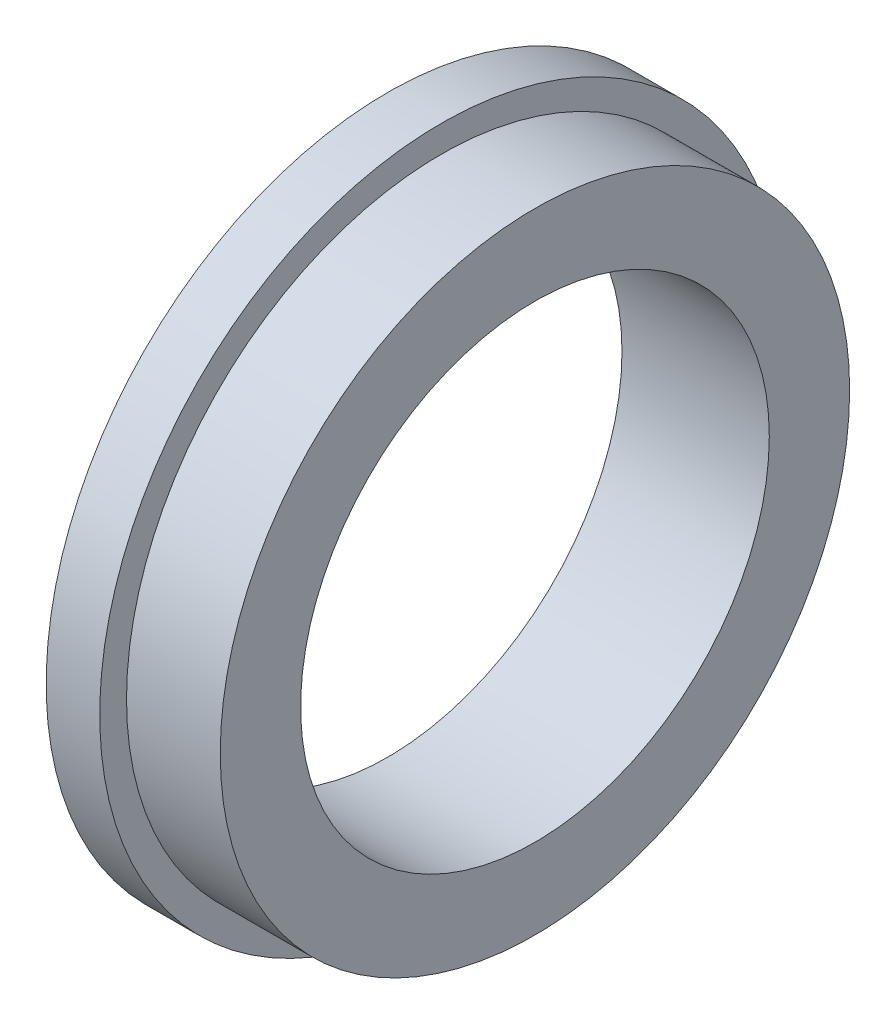
SolidWorks part; units mm, degrees
ref_plane "Front" through (0, 0, 0) normal (0, 0, 1) x (1, 0, 0)
ref_plane "Top" through (0, 0, 0) normal (0, 1, 0) x (1, 0, 0)
ref_plane "Right" through (0, 0, 0) normal (1, 0, 0) x (0, 0, -1)
sketch "Sketch1" plane through (0, 0, 0) normal (0, 0, 1) x (1, 0, 0)
  line L0 (-7.229, 17.5) -> (3.771, 17.5)
  line L1 (3.771, 17.5) -> (3.771, 23.5)
  line L2 (3.771, 23.5) -> (-3.229, 23.5)
  line L3 (-3.229, 23.5) -> (-3.229, 25.5)
  line L4 (-3.229, 25.5) -> (-7.229, 25.5)
  line L5 (-7.229, 25.5) -> (-7.229, 17.5)
  line L6 (0, 0) -> (-60.9414, 0) construction
  dimension "D1" = 17.5
  dimension "D2" = 11
  dimension "D3" = 8
  dimension "D4" = 4
  dimension "D5" = 2
revolve "Revolve1" add sketch "Sketch1" angle 360 about L6
scale "Scale 1" bodies to scale 101 scale about centroid uniform scaling yes scale factor 1.875
